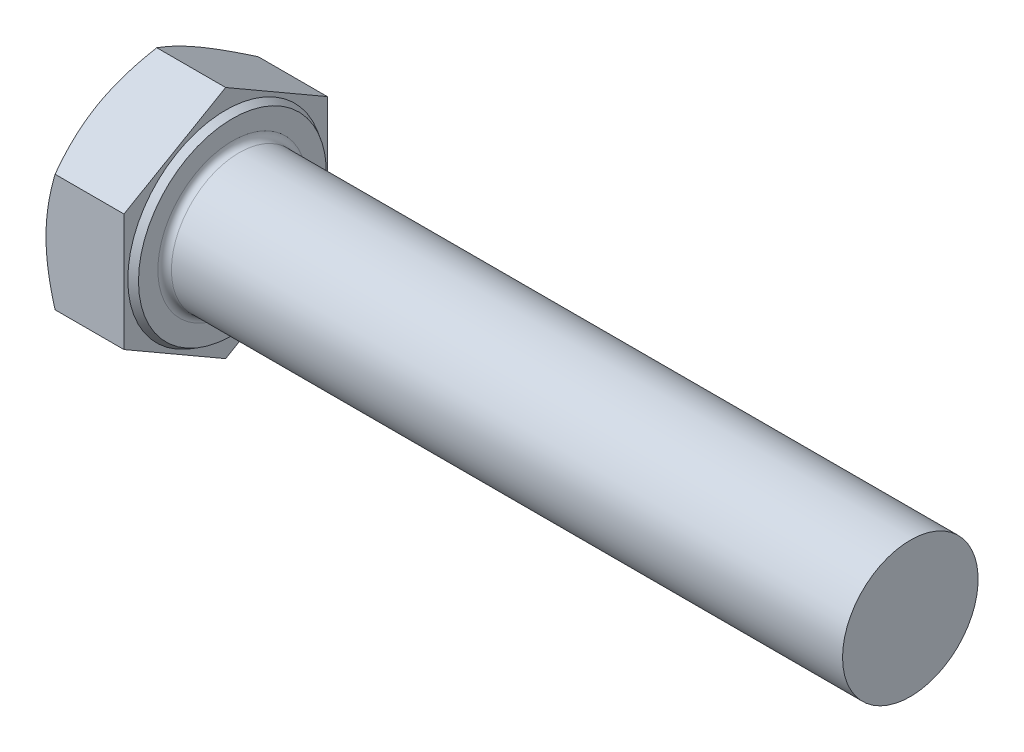
SolidWorks part; units mm, degrees
ref_plane "前视" through (0, 0, 0) normal (0, 0, 1) x (1, 0, 0)
ref_plane "上视" through (0, 0, 0) normal (0, 1, 0) x (1, 0, 0)
ref_plane "右视" through (0, 0, 0) normal (1, 0, 0) x (0, 0, -1)
sketch "草图1" plane through (0, 0, 0) normal (1, 0, 0) x (0, 0, -1)
  line L0 (9, 5.1962) -> (9, -5.1962)
  line L1 (-9, 5.1962) -> (-9, -5.1962)
  line L2 (9, -5.1962) -> (0, -10.3923)
  line L3 (0, -10.3923) -> (-9, -5.1962)
  line L4 (9, 5.1962) -> (0, 10.3923)
  line L5 (0, 10.3923) -> (-9, 5.1962)
  circle A0 centre (0, 0) radius 10.015 construction
  dimension "e" = 20.03
  dimension "s" = 18
  dimension "D2" = 120
  dimension "D3" = 9
  dimension "D4" = 9
  dimension "D5" = 9
extrude "基体-拉伸" add sketch "草图1" along normal blind 7.5
sketch "草图2" plane through (0, 0, 0) normal (0, 0, 1) x (1, 0, 0)
  line L0 (0, 5.1962) -> (0, -5.1962) construction
  line L1 (0, 0) -> (67.5, 0)
  line L2 (0, 0) -> (0, 6)
  line L3 (0, 6) -> (37.5, 6)
  line L4 (67.5, 0) -> (67.5, 4.4845)
  line L5 (7.5, 10.3923) -> (7.5, 5.1962) construction
  line L7 (0, 0) -> (79.5, 0) construction
  line L8 (67.5, -4.4845) -> (37.5, -6) construction
  line L9 (0, -6) -> (37.5, -6) construction
  line L10 (9.25, 6) -> (9.25, 0) construction
  line L11 (37.5, 15.24) -> (37.5, -1.27) construction
  line L12 (7.5, 5.1962) -> (7.5, -5.1962) construction
  line L13 (37.5, 6) -> (67.5, 6)
  line L14 (67.5, 6) -> (67.5, 4.4845)
  dimension "l" = 60
  dimension "d" = 12
  dimension "Minor_dia" = 8.969
  dimension "p" = 1.75
  dimension "b" = 30
  dimension "ds" = 12
revolve "凸台-旋转1" add sketch "草图2" angle 360 about L7
cosmetic thread "螺旋线1" parameters "Thread_length"=30, "Thread_minor"=8.969
sketch "草图3" plane through (0, 0, 0) normal (0, 0, 1) x (1, 0, 0)
  line L0 (0, 9) -> (3.6906, 15.3923)
  line L1 (0, 10.3923) -> (0, 5.1962) construction
  line L2 (3.6906, 15.3923) -> (3.6906, 20.3923)
  line L3 (3.6906, 20.3923) -> (-10, 20.3923)
  line L4 (-10, 20.3923) -> (-10, 9)
  line L5 (-10, 9) -> (0, 9)
  line L6 (0, 0) -> (99.06, 0) construction
  line L7 (7.5, 10.3923) -> (0, 10.3923) construction
  dimension "D1" = 9
  dimension "D2" = 5
  dimension "D3" = 10
  dimension "D4" = 5
  dimension "Head_ch_ang" = 30
revolve "切除-旋转1" cut sketch "草图3" angle 360 about L6
sketch "草图4" plane through (0, 0, 0) normal (0, 0, 1) x (1, 0, 0)
  line L0 (7.5, 0) -> (7.5, 8.315) construction
  line L2 (7.5, -6) -> (7.5, 6) construction
  line L3 (7.5, 10.3923) -> (7.5, 5.1962) construction
  line L4 (7.5, 8.315) -> (6.9, 8.6614)
  line L5 (0, 0) -> (95.25, 0) construction
  line L6 (0, 0) -> (79.5, 0) construction
  line L9 (6.9, 8.6614) -> (6.9, 10.3923)
  line L10 (7.5, 10.3923) -> (0.8038, 10.3923) construction
  line L11 (6.9, 10.3923) -> (7.5, 10.3923)
  line L12 (7.5, 10.3923) -> (7.5, 8.315)
  dimension "D1" = 120
  dimension "c" = 0.6
  dimension "dw" = 16.63
revolve "切除-旋转3" cut sketch "草图4" angle 360 about L5
fillet "圆角" radius 0.6 1 edges at (7.5, 0, -6)
sketch "草图6" plane through (0, 0, 0) normal (0, 0, 1) x (1, 0, 0)
  line L0 (0, 0) -> (67.5, 0) construction
  line L1 (67.5, -6) -> (67.5, 6) construction
  line L2 (67.5, 0) -> (67.5, 6) construction
  line L4 (66.625, 6) -> (68.375, 6)
  line L5 (66.625, 6) -> (67.5, 4.4845)
  line L6 (67.5, 4.4845) -> (68.375, 6)
  dimension "D1" = 1.75
revolve "切除-旋转4" [suppressed] cut sketch "草图6" angle 360 about L0
pattern_linear "阵列(线性)1" [suppressed]
